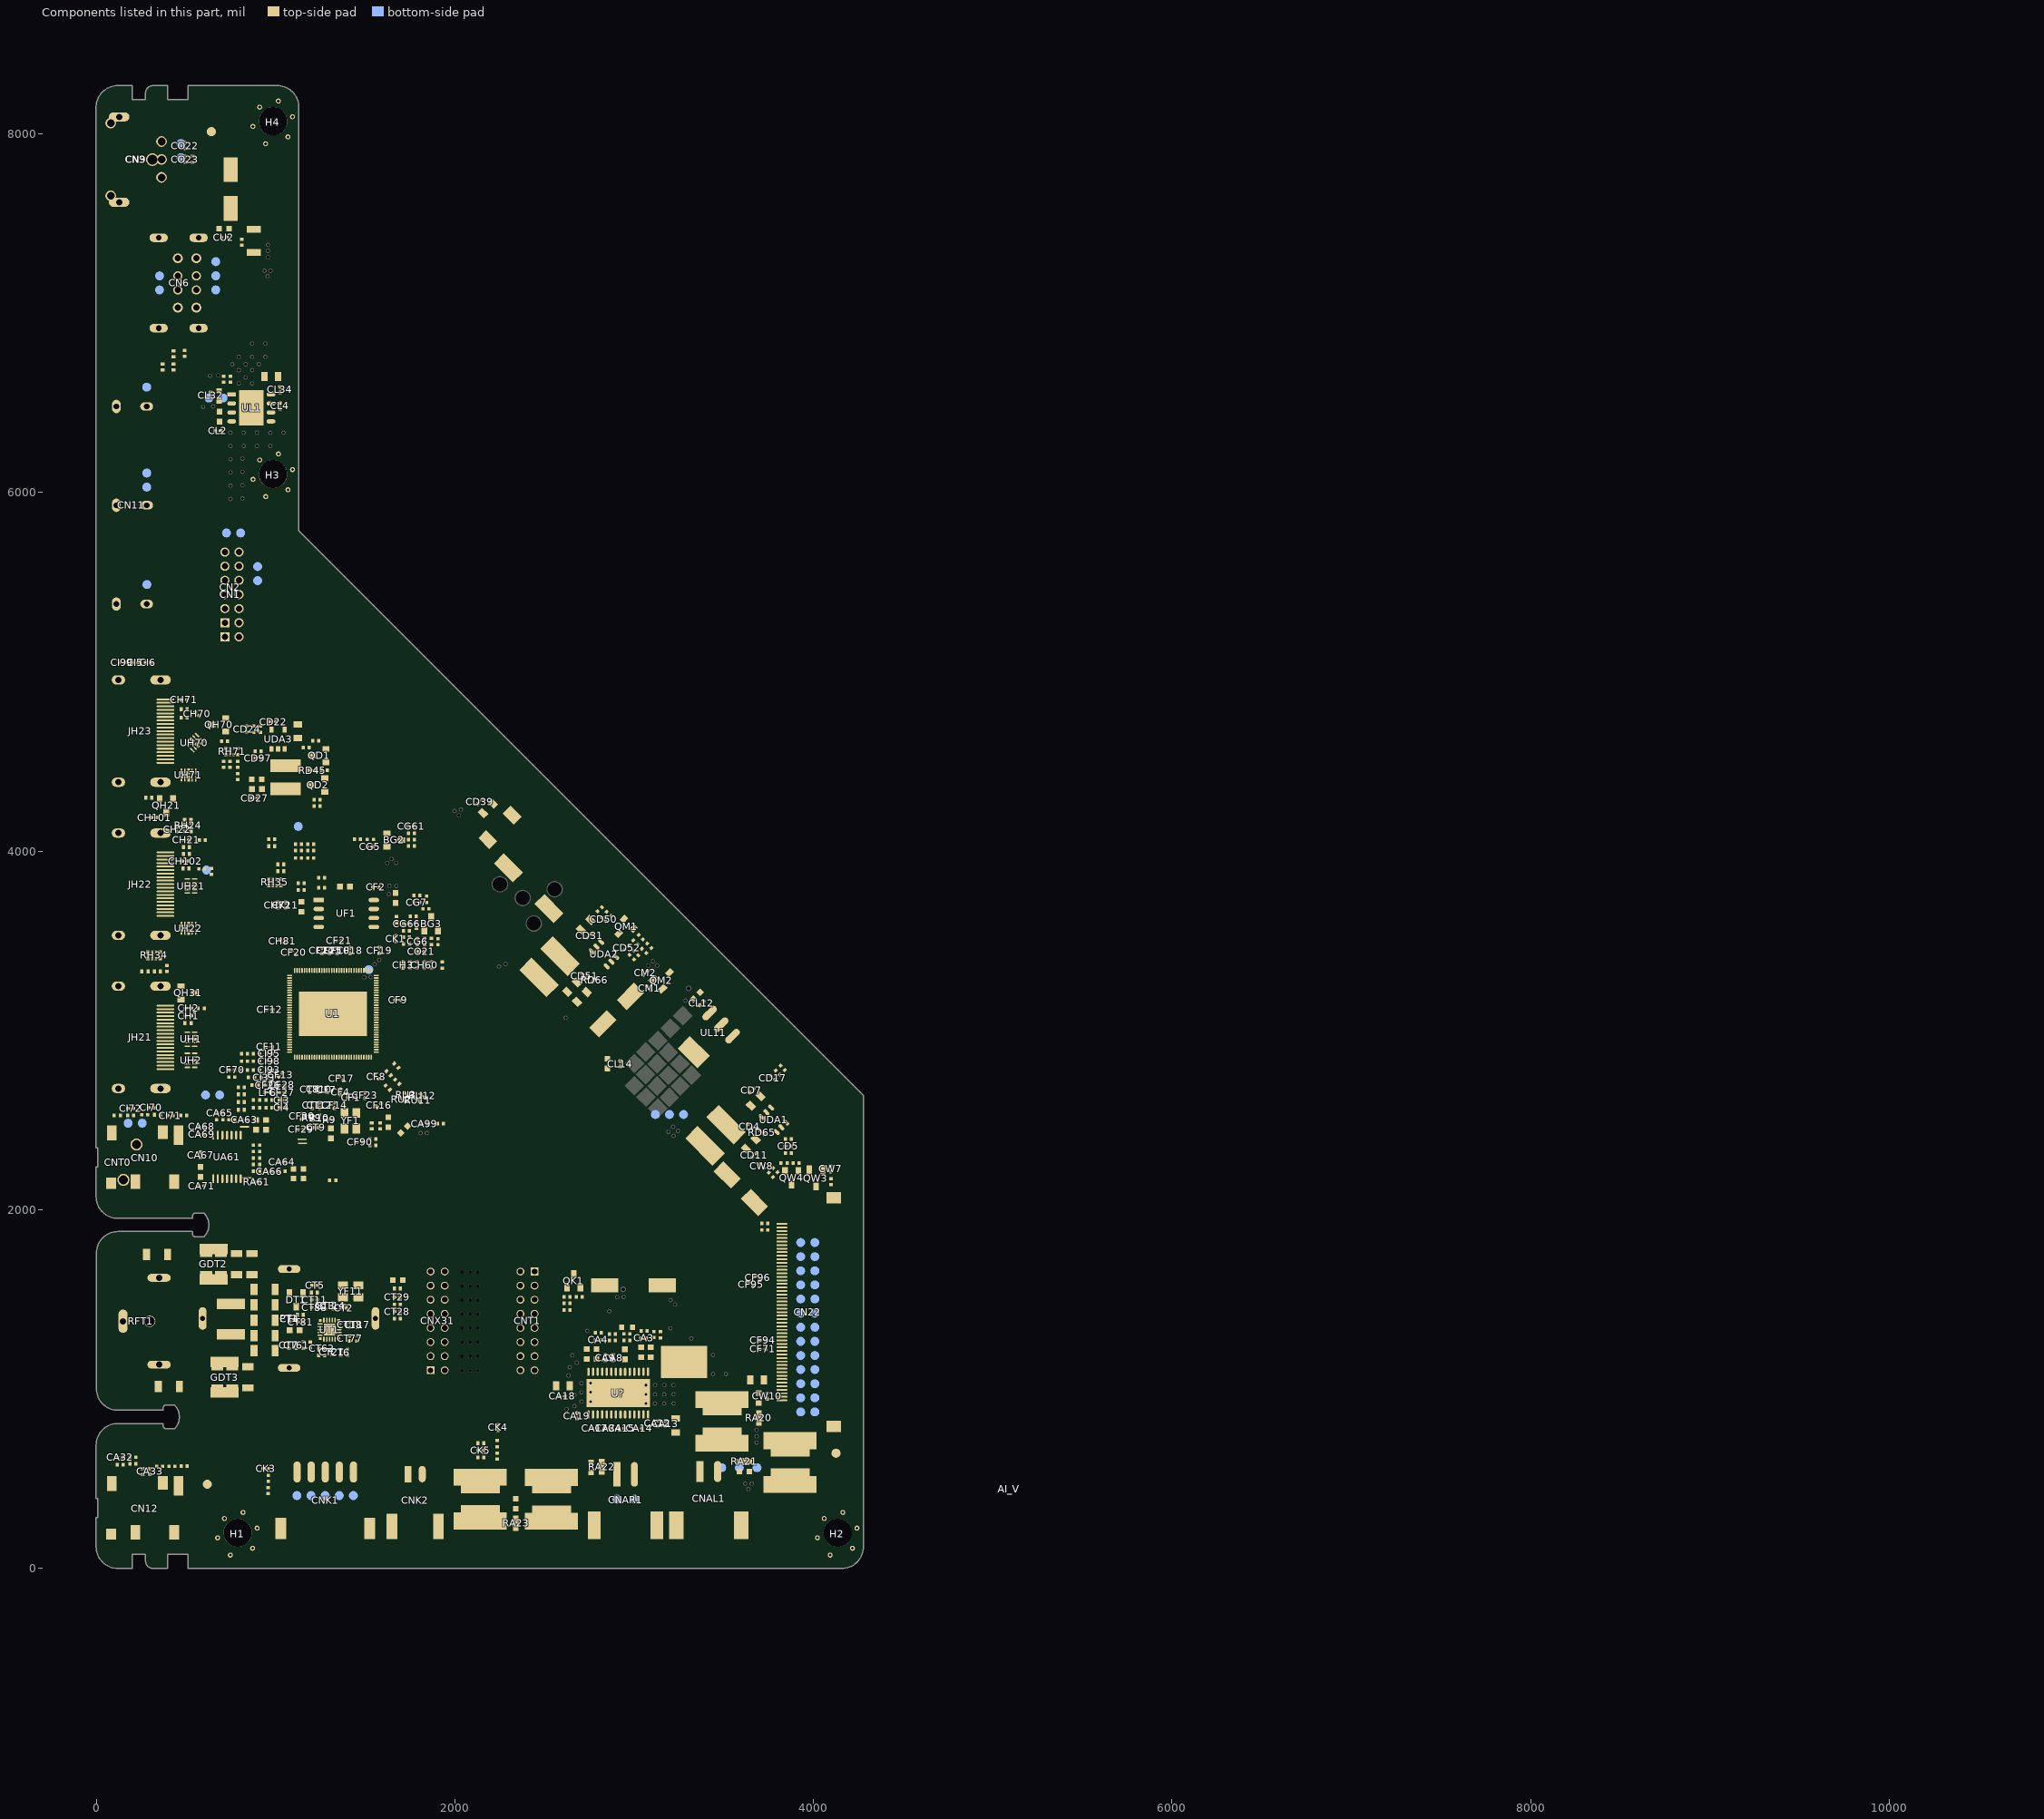
[diagram p0: the components of this part, seen from the top]
# Altium PCB MISC105950.PcbDoc (part 14 of 15)
Units mil, origin at the board's own origin, x right, y up, seen from the top; angles counter-clockwise.
Board outline 4280.62 x 8272.76 mil, 2 copper layers (TopLayer, BottomLayer), stack 61.855 mil thick; 541 components, 268 nets, 2324 pads, 1157 vias.

## Via types
v1: diameter 23.62, hole 15.75, TopLayer to BottomLayer, tented both sides, 1087 vias
v2: diameter 23.62, hole 15.75, TopLayer to BottomLayer, 51 vias
v3: diameter 27.56, hole 19.68, TopLayer to BottomLayer, 15 vias
v4: diameter 31.5, hole 19.68, TopLayer to BottomLayer, tented both sides, 4 vias

## Nets (pads, with @x,y where several pads share a name; then routed paths per layer and width w, separated by ;. In a path a pad name is that pad's centre, name@x,y a point inside that pad or via, vN(x,y) a via of type N, cw(c..) or ccw(c..) an arc to the next point about the centre after c; other vN are vias at no path point) (continued)
pads on no net: AI_V.0 AI_V.1 AI_V.2 CA3.2@3053,1282.5 CA4.2@2799.03,1273.23 CA8.2@2881.84,1172.5 CA9.2@2837.44,1172.5 CA12.2@3130.5,806.5 CA13.2@3173,806.16 CA14.2@3027,779 CA15.2@2929,779 CA17.2@2781,779 CA18.2@2598.5,958.5 CA19.2@2680,848.5 CA32.2@131.5,617 CA33.2@297,538.5 CA34.2@2855.5,779 CA63.2@824.76,2501 CA64.2@1035,2266 CA65.2@688,2539.5 CA66.2@962.73,2213.5 CA67.2@580,2304 CA68.2@585.66,2461.68 CA69.2@585.66,2420 CA71.2@585.34,2131.5 CA99.2@1829.34,2478.5 CD4.2@3643.54,2463.96 CD5.2@3858.27,2353.5 CD7.2@3654.54,2664.04 CD11.2@3669.5,2303.5 CD17.2@3773.5,2734.5 CD22.2@984.66,4721.5 CD24.2@838,4680.5 CD27.2@882.16,4295.5 CD31.2@2749,3527.51 CD39.2@2138.5,4274.5 CD50.2@2829,3619 CD51.2@2721.51,3302 CD52.2@2956.72,3460.11 CD97.2@900.77,4517.5 CF1.2@1417.66,2625 CF2.2@1558,3798 CF4.2@1361.5,2655.66 CF7.2@1285.5,2668.16 CF8.2@1561.5,2741.5 CF9.2@1681.5,3168.5 CF10.2@1341.5,3444.33 CF11.2@963.27,2907 CF12.2@965.5,3115.5 CF13.2@1026.5,2752 CF14.2@1326.5,2580.74 CF16.2@1575.96,2581.46 CF17.2@1365.5,2731.5 CF18.2@1414,3444.5 CF19.2@1577,3446 CF20.2@1099.67,3434.33 CF21.2@1352.16,3500.5 CF23.2@1497,2637.5 CF24.2@1257,3444.33 CF25.2@1299.5,3444.34 CF26.2@956,2693.5 CF27.2@1035,2652.5 CF28.2@1035,2694.5 CF29.2@1139.5,2447 CF30.2@1144.5,2520.23 CF70.2@755,2778 CF71.2@3716.5,1221.48 CF90.2@1469,2377 CF94.2@3716.5,1270.18 CF95.2@3650.86,1582.02 CF96.2@3688.61,1619.48 CG5.2@1525.5,4024 CG6.2@1789.5,3495.5 CG7.2@1786,3714 CG61.2@1754,4138.5 CG66.2@1729,3595 CH1.2@512.5,3081 CH2.2@512.5,3123 CH3.2@1709.5,3363.5 CH21.2@500.34,4062.1 CH22.2@449.5,4121.5 CH60.2@1828.5,3364.5 CH70.2@561.52,4764.99 CH71.2@488.5,4843.5 CH72.2@1011.5,3698.39 CH81.2@1037,3497 CH101.2@322.66,4187.5 CH102.2@493.83,3943.6 CI3.2@1034.99,2610 CI4.2@1034.99,2568 CI5.2@217,5052 CI6.2@288.5,5052 CI33.2@935.5,2736.5 CI70.2@305,2568.5 CI71.2@411,2524.5 CI72.2@190.5,2564 CI93.2@963.5,2778.5 CI95.2@963.5,2869 CI98.2@963.5,2827.5 CI99.2@143.5,5052 CK1.2@1670,3511 CK3.2@945,554.5 CK4.2@2240,784.5 CK5.2@2143,656.5 CK11.2@1053.5,3698.4 CL2.2@678,6345 CL4.2@1023.5,6483 CL12.2@3376,3150.5 CL14.2@2921.5,2813 CL32.2@635.42,6543.27 CL34.2@1023.5,6574.5 CM1.2@3082.7,3234.09 CM2.2@3061.5,3320 CN1.0 CN1.9 CN2.0 CN2.7 CN3.0 CN6.0 CN9.0 CN10.0 CN11.0 CN12.0 CN22.5 CN22.9 CN22.10 CN22.25 CN22.26 CN22.42 CN22.43 CN22.44 CN22.46 CN22.47 CN22.48 CN22.49 CN22.50 CN22.51 CNT0.0 CNT0.1 CNT1.0 CNT1.8 CNX31.0 CNX31.10 CO21.2@1811,3438.5 CO22.2@493,7935.37 CO23.2@493,7858.88 CT1.2@1201.5,2581.73 CT2.2@1377,1451 CT3.2@1276,1463 CT4.2@1077.5,1390.5 CT5.2@1217.5,1577 CT6.2@1361.5,1203.5 CT7.2@1072.5,1242.5 CT8.2@1189,2669.5 CT9.2@1223.34,2457 CT10.2@1241,2669.5 CT11.2@1214.98,1496.39 CT12.2@1244,2581.73 CT14.2@1318,1463 CT17.2@1455,1357.5 CT18.2@1412.5,1357.5 CT21.2@1313,1205.5 CT28.2@1678,1431.5 CT29.2@1677,1510.5 CT61.2@1114.5,1242.5 CT62.2@1256.5,1224.5 CT77.2@1412.5,1281.5 CT81.2@1137,1372.5 CT88.2@1214.99,1453.9 CU2.2@711,7423.88 CW7.2@4095.5,2227 CW8.2@3710.76,2241.97 CW10.2@3741.5,959 GDT2.1@613,1635.93 GDT2.1@654.98,1596.61 GDT2.1@693,1635.93 GDT2.2@613,1754.07 GDT2.2@654.98,1793.39 GDT2.2@693,1754.07 GDT3.1@674.5,1123.07 GDT3.1@712.52,1162.39 GDT3.1@754.5,1123.07 GDT3.2@674.5,1004.93 GDT3.2@712.52,965.61 GDT3.2@754.5,1004.93 H1.0 H2.0 H3.0 H4.0 JH21.0 JH22.0 JH23.0 JH23.14 M1.0 M2.0 M3.0 Manufacture_Info.0 PT1.0 RFT1.0 S/N1.0 S/N2.0 U1.0 U?.13 U?.EPAD UT1.1 UT1.9 UT1.10 UT1.15 XX.XXXX.0 XXXXXX.0 XXXXXX..0 XXXXXXXX.0 XXXXXXXXXX.0 用U1上.0
copper on no net: | length 3400.6
  TopLayer w5: 8224.49,3310.69 8224.49,3389.43 ; 7673.59,3310.69 8405.62,3310.69 8405.62,3389.43 7673.59,3389.43 7673.59,3310.69
  BottomLayer w5: 8224.49,3092.84 8224.49,3171.58 ; 7673.59,3092.84 7673.59,3171.58 8405.62,3171.58 8405.62,3092.84 7673.59,3092.84
  other v1: 2737.24,898.49 2816.34,898.27 2879.33,898.27 2942.33,898.27 3006.33,898.27 3083.17,898.49 2737.24,936.95 3083.17,936.95 2737.24,975.41 3083.17,975.41 2737.24,1013.86 3083.17,1013.86 2737.24,1052.32 2816.34,1052.09 2879.33,1052.09 2942.33,1052.09 3006.33,1052.1 3083.17,1052.32
  other v3: 2783.2,922.26 2847.21,922.26 2910.2,922.26 2973.2,922.26 3037.2,922.26 2783.2,975.41 2847.21,975.41 2910.2,975.41 2973.2,975.41 3037.2,975.41 2783.2,1028.56 2847.21,1028.56 2910.2,1028.56 2973.2,1028.56 3037.2,1028.56

## Polygon pours and split planes (outlines as drawn)
GND on BottomLayer "5" (solid, remove dead copper, pour order 22): 1135.5,5505 1092,5461.5 883.5,5461.5 883,5461.5 853.5,5432 853.5,5368 897,5324.5 897,5074.5 873.5,5051 541,4718.5 541,4636 345,4636 168,4459 168,2786 467,2487 768,2487 951.5,2303.5 1112.5,2142.5 1112.5,2074 1151.5,2074 1204.5,2021 1650.83,2021 1680.17,2050.33 1734.5,2104.67 1734.5,2170.5 1781.5,2217.5 2038,2217.5 2203.5,2052 2203.5,1699.5 2203.5,898 2249.5,852 2339.5,852 2774,1286.5 2774,1449 2852,1527 2852,1535.65 2875.58,1559.22 2900.35,1584 2946.5,1584 2987,1584 3093.5,1690.5 3121,1718 3121,1758.5 3121,2412.67 3170.16,2461.83 3159.5,2472.49 3159.5,2570 3159.5,2648.5 3296,2785 3395.5,2685.5 3454.5,2685.5 3454.5,2649.5 3751,2353 3849,2451 3951.5,2451 3951.5,2689 3959,2696.5 1161.5,5494 1161.5,5525
GND on BottomLayer "5" (solid, remove dead copper, pour order 23): 1873,2503.5 1745.5,2503.5 1725,2524 1703,2546 1703,2573 1703,2595 1732,2624 1734,2626 1779,2626 1782,2626 1810.5,2654.5 2029,2873 2029,3070.5 2029,3447 2124.5,3542.5 2146.31,3564.31 2216.93,3564.31 2277.5,3503.74 2277.5,3441 2277.5,3404.5 2254,3381 2202.5,3381 2190.5,3369 2181.5,3360 2181.5,3238 2181.5,2834 2038,2690.5 1945.67,2598.17 1945.67,2572 1945.67,2544.19 1928.79,2527.31 1904.98,2503.5 1873,2503.5
RFGND on BottomLayer "12" (solid, remove dead copper, pour order 18): 217.5,1908 71,1908 -6.5,1830.5 -6.5,929 56,866.5 271,866.5 328,923.5 467.5,1063 606.5,1063 890,1063 936.5,1109.5 936.5,1652.5 904,1685 465,1685 394.5,1755.5 273,1877 268,1877
GND on BottomLayer "12" (solid, remove dead copper, pour order 19): 67.5,2492.5 1238,2492.5 1750,1980.5 1750,1235 1127,612 1115.5,600.5 815.5,600.5 381,600.5 298.5,683 298.5,878.5 459,1039 873,1039 938,1104 938,1663 928,1673 458,1673 301,1830 225,1906 -57,1906 -57,1966.5 -171,2080.5
GND on BottomLayer "12" (solid, remove dead copper, pour order 20): 596.5,8267.72 100,8267.72 ccw(c100,8167.72) 0,8167.72 0,8129 0,2053.33 ccw(c100,2053.33) 100,1953.33 294,1953.33 294,1852 443.5,1702.5 903.82,1702.5 948.07,1658.25 948.07,1124.07 900,1076 482.5,1076 382.5,976 199,792.5 172,792.5 82.92,792.5 ccw(c82.92,692.5) 12.21,763.21 2,753 ccw(c11.66,743.34) -2,743.34 -2,644.5 -2,100 ccw(c98,100) 98,0 145.5,0 4173.75,0 ccw(c4173.75,100) 4273.75,100 4273.75,334.08 4273.75,2638.25 4101.5,2810.5 1125.98,5786.02 1125.98,6061 1125.98,8167.78 ccw(c1025.98,8167.78) 1025.98,8267.78 994,8267.78 553.5,8267.78
GND on BottomLayer "5" (solid, remove dead copper, pour order 21): 4064.5,1940 3740.5,1940 3633,1832.5 3637,1828.5 3637,1821 3637,1041 3932,746 3940.5,737.5 4103.5,737.5 4103.5,838.5 4140.5,875.5 4130,886 4130,1964.5
GND on TopLayer "12" (solid, remove dead copper, pour order 15): 596.5,8267.72 100,8267.72 ccw(c100,8167.72) 0,8167.72 0,8129 0,2053.33 ccw(c100,2053.33) 100,1953.33 294,1953.33 294,1852 443.5,1702.5 903.82,1702.5 948.07,1658.25 948.07,1124.07 900,1076 482.5,1076 382.5,976 199,792.5 172,792.5 82.92,792.5 ccw(c82.92,692.5) 12.21,763.21 2,753 ccw(c11.66,743.34) -2,743.34 -2,644.5 -2,100 ccw(c98,100) 98,0 145.5,0 4173.75,0 ccw(c4173.75,100) 4273.75,100 4273.75,334.08 4273.75,2638.25 4101.5,2810.5 1125.98,5786.02 1125.98,6061 1125.98,8167.78 ccw(c1025.98,8167.78) 1025.98,8267.78 994,8267.78 553.5,8267.78
RFGND on TopLayer "12" (solid, remove dead copper, pour order 17): 889.86,1695.63 468.87,1695.63 343,1821.5 271,1893.5 72,1893.5 38,1893.5 18,1873.5 1.21,1856.71 1.21,1532.5 1.21,910.79 40.5,871.5 51.47,882.47 219,882.47 315.97,882.47 365.5,932 481.5,1048 695.5,1048 882.5,1048 924.5,1090 938,1103.5 938,1574 938,1650.71 943.75,1656.46 904.59,1695.63 889.86,1695.63
GND on TopLayer "5" (solid, remove dead copper, pour order 16): 507,4715.33 449.83,4715.33 435.5,4701 435.5,4456.5 442.5,4449.5 442.5,4303.5 485.5,4260.5 670.66,4075.34 670.66,3880 669,3880 657.5,3868.5 652.56,3863.56 448.47,3863.56 444.4,3863.56 435.16,3854.33 435.16,3636.84 423,3624.68 423,3623.88 431.33,3615.56 452.48,3594.41 452.48,3564.5 452.48,3467.89 557.59,3362.78 652,3268.37 652,3120 652,3076.36 598.64,3023 586.52,3010.88 462.88,3010.88 446.04,3010.88 435.16,3000 435.16,2774.01 431,2769.85 433.03,2771.87 487,2771.87 640.69,2771.87 690.81,2822 775.81,2907 785,2907 884,2907 885.5,2905.5 956.47,2905.5 999.83,2948.86 1056.5,3005.53 1056.5,3084.99 1056.5,3291.04 1087.25,3321.79 1099.49,3334.04 1104.92,3334.04 1126.19,3355.31 1126.19,3379.5 1126.19,3392.5 1126.19,3407.81 1048.83,3485.17 1048.83,3498.73 1009.14,3538.42 883.5,3664.07 883.5,3858.5 883.5,4213.48 880,4216.98 866.84,4230.14 866.84,4235.3 709.78,4392.36 676.33,4392.36 676.33,4560.95 623.51,4613.76 515.6,4721.67 485.37,4721.67
GND on TopLayer "5" (solid, remove dead copper, pour order 13): 342.07,7337 306.59,7337 111.81,7142.22 111.81,6802.69 225.5,6689 288,6689 320.5,6656.5 320.5,5075.04 615.04,4780.5 1108,4780.5 1251.21,4637.29 1343.99,4637.29 1396.69,4584.6 1402.81,4584.6 1402.81,4542.19 1771,4174 1833.53,4174 2046.76,3960.76 2046.76,3749.24 2089,3707 2089,3479 2158.5,3409.5 2247,3409.5 2259,3421.5 2259,3680.5 2159,3780.5 2159,3993.67 1203.17,4949.5 648.5,4949.5 475,5123 475,6580 527,6632 527,6820.5 500,6847.5 293.5,6847.5 254,6887 254,7047.43 258.66,7052.09 336.09,7052.09 375,7091 375,7317 354.56,7337.44 341.44,7337.44
GND on TopLayer "5" (solid, remove dead copper, pour order 14): 1633.94,3293.19 1633.94,3279.02 1576.5,3221.58 1576.5,2893.5 1563,2880 1541.36,2880 1536.17,2885.18 1504.52,2853.54 1504.52,2793.64 1602.83,2695.33 1602.83,2688.57 1769.93,2521.47 1948.68,2521.47 1963.3,2506.84 2069.97,2506.84 2167.89,2408.92 2205.25,2408.92 2813.45,1800.72 2899.78,1800.72 3045.5,1655 3057.5,1655 3057.5,1625.7 3102.95,1580.24 3102.95,1502.55 3122.96,1522.55 3235.95,1522.55 3657.06,1101.44 3703.5,1101.44 3716.44,1088.5 3762,1088.5 3778.96,1071.54 3778.96,1014.84 3800.66,1014.84 3870,945.5 4003,945.5 4116.5,1059 4116.5,1751.5 3996.5,1871.5 3918.42,1871.5 3865.85,1818.93 3865.85,1741.35 3845.5,1721 3796.61,1721 3781.9,1735.71 3783.63,1737.44 3783.63,1801.37 3775.5,1809.5 3775.5,1839.45 3754.93,1860.03 3720.71,1860.03 3224.59,2356.15 3145.35,2356.15 2267.1,3234.4 2213.19,3234.4 2171.88,3275.72 2129.78,3275.72 2068.2,3337.3 1968.03,3337.3 1951.23,3320.5 1645.25,3320.5 1633.94,3309.19 1633.94,3293.19

## Keep-outs
KeepOutLayer:
  circle w2.5: c118.11,8267.73 r1.25
  circle w2.5: c4275.59,118.11 r1.25
  circle w2.5: c1185.04,8326.78 r1.25
  circle w2.5: c5342.52,177.16 r1.25
  rectangle: 7673.59,2713.41 7803.79,2792.15
  lines w5: 0,2346 7.42,2346 7.87,2345.54 7.87,2236.22 0,2236.22 0,2071.44 ccw(c118.11,2071.44) 118.11,1953.33 532,1953.33 ; 0,2346.46 0,8153 ; 0,8149.62 cw(c118.11,8149.62) 118.11,8267.73 196.85,8267.73 196.85,8188.99 275.59,8188.99 275.59,8228.36 cw(c314.96,8228.36) 314.96,8267.73 393.7,8267.73 393.7,8188.99 511.81,8188.99 511.81,8267.73 1008.03,8267.72 ; 368.5,803.73 118.11,803.73 ccw(c118.11,685.62) 0,685.62 0,389.76 7.87,389.76 7.87,279.53 0,279.53 0,118.11 ccw(c118.11,118.11) 118.11,0 196.85,0 196.85,78.74 275.59,78.74 275.59,39.37 ccw(c314.96,39.37) 314.96,0 393.7,0 393.7,78.74 511.81,78.74 511.81,0 4157.48,0 ccw(c4157.48,118.11) 4275.59,118.11 4275.59,2576.35 4275.59,2635.41 1125.98,5785.02 1125.98,8149.61 ccw(c1007.87,8149.61) 1007.87,8267.72 ; 368.5,882.47 119.32,882.47 cw(c119.32,1000.58) 1.21,1000.58 1.21,1756.48 cw(c119.32,1756.48) 119.32,1874.59 532,1874.59 ; 368.7,803.32 368.7,793.82 ccw(c388.39,793.82) 388.39,774.14 436.03,774.14 ccw(c367.13,843.03) 436.03,911.93 388.39,911.93 ccw(c388.39,892.25) 368.7,892.25 368.7,882.47 ; 396.88,2108.85 235.46,2108.85 ; 532.7,1874.59 532.7,1864.75 ccw(c552.39,1864.75) 552.39,1845.07 600.03,1845.07 ccw(c531.13,1913.96) 600.03,1982.86 552.39,1982.86 ccw(c552.39,1963.18) 532.7,1963.18 532.7,1953.33 ; 640.2,774.14 687.84,774.14 ccw(c618.94,843.03) 687.84,911.93 640.2,911.93 ; 642.72,774.14 595.08,774.14 cw(c663.98,843.03) 595.08,911.93 642.72,911.93 ; 708.54,8267.72 ccw(c679.01,8297.25) 708.54,8326.78 ; 826.41,1874.59 826.41,1864.75 cw(c806.72,1864.75) 806.72,1845.07 759.08,1845.07 cw(c827.98,1913.96) 759.08,1982.86 806.72,1982.86 cw(c806.72,1963.18) 826.41,1963.18 826.41,1953.33 ; 826.5,1874.59 1922.47,1874.59 cw(c1922.47,1756.48) 2040.58,1756.48 2040.58,1740 ; 826.5,1953.33 2048.46,1953.33 cw(c2048.46,1874.59) 2127.2,1874.59 ; 914.22,803.71 914.22,793.82 cw(c894.53,793.82) 894.53,774.14 846.89,774.14 cw(c915.79,843.03) 846.89,911.93 894.53,911.93 cw(c894.53,892.25) 914.22,892.25 914.22,882.46 ; 915.5,803.71 2048.44,803.71 ccw(c2048.46,882.47) 2127.2,882.47 2126.93,882.74 2126.93,1016.5 ccw(c2083.78,973.35) 2040.63,1016.5 2040.58,1000.5 ; 915.5,882.47 1922.47,882.47 ; 993.88,8267.72 cw(c1023.41,8297.25) 993.88,8326.78 ; 1125.98,7500.79 cw(c1155.51,7471.26) 1185.04,7500.79 ; 1125.99,7943.61 ccw(c1155.51,7973.14) 1185.04,7943.61 ; 1662.12,5248.86 ccw(c1662.12,5290.62) 1703.88,5290.62 ; 1670.27,5324.25 3408.51,3586.01 ; 1753.78,5157.22 3467.62,3443.38 ; 1975.24,4935.74 cw(c2017,4935.74) 2017,4977.5 ; 2040.63,1740.57 ccw(c2083.78,1783.72) 2126.93,1740.57 2127.2,1740.84 2127.2,1769.74 ; 3412.18,7641.16 ccw(c3412.18,7562.42) 3333.44,7562.42 3333.44,6675.15 3333.44,6570.29 ccw(c3412.18,6570.29) 3412.18,6491.55 4870.45,6491.55 4870.45,6481.71 ccw(c4890.13,6481.71) 4890.13,6462.02 4937.77,6462.02 ccw(c4868.87,6530.92) 4937.77,6599.82 4890.13,6599.82 ccw(c4890.13,6580.13) 4870.45,6580.13 4870.45,6570.29 3538.16,6570.29 cw(c3538.16,6688.4) 3420.05,6688.4 3420.05,7444.31 ; 3412.19,7641.17 4870.45,7641.17 4870.45,7651.06 cw(c4890.13,7651.06) 4890.13,7670.75 4937.77,7670.75 cw(c4868.87,7601.85) 4937.77,7532.95 4890.13,7532.95 cw(c4890.13,7552.64) 4870.45,7552.64 4870.45,7562.43 ; 3420.05,7444.39 cw(c3538.16,7444.31) 3538.16,7562.42 4870.45,7562.42 ; 3443.63,3467.39 ccw(c3443.63,3509.14) 3485.39,3509.14 ; 3756.75,3154.27 cw(c3798.51,3154.27) 3798.51,3196.02 ; 4275.59,501.28 cw(c4305.12,471.75) 4334.65,501.28 ; 4275.59,944.1 ccw(c4305.12,973.62) 4334.65,944.1 ; 4452.6,177.17 4948.82,177.17 4948.82,255.9 5066.93,255.9 5066.93,177.16 5145.67,177.16 ccw(c5145.67,216.53) 5185.04,216.53 5185.04,255.9 5263.78,255.9 5263.78,177.16 5342.52,177.16 ccw(c5342.52,295.27) 5460.63,295.27 ; 4452.76,177.17 cw(c4452.76,295.28) 4334.65,295.28 4334.65,2659.87 1185.04,5809.48 1185.04,5868.53 1185.04,8326.78 cw(c1303.15,8326.78) 1303.15,8444.89 4948.82,8444.89 4948.82,8366.15 5066.93,8366.15 5066.93,8444.89 5145.67,8444.89 cw(c5145.67,8405.52) 5185.04,8405.52 5185.04,8366.15 5263.78,8366.15 5263.78,8444.89 5342.52,8444.89 cw(c5342.52,8326.78) 5460.63,8326.78 5460.63,8165.36 5452.76,8165.36 5452.76,8055.12 5460.63,8055.12 5460.63,7759.27 cw(c5342.52,7759.27) 5342.52,7641.16 5164.13,7641.16 ; 4466.76,118.11 ccw(c4437.23,147.64) 4466.76,177.17 ; 4752.09,118.11 cw(c4781.62,147.64) 4752.09,177.17 ; 5164.15,6491.55 5164.15,6481.71 cw(c5144.46,6481.71) 5144.46,6462.02 5096.83,6462.02 cw(c5165.72,6530.92) 5096.83,6599.82 5144.46,6599.82 cw(c5144.46,6580.13) 5164.15,6580.13 5164.15,6570.29 5341.31,6570.29 ccw(c5341.31,6688.4) 5459.42,6688.4 5459.42,7444.31 ccw(c5341.31,7444.31) 5341.31,7562.42 5164.15,7562.42 5164.15,7552.64 cw(c5144.46,7552.64) 5144.46,7532.95 5096.83,7532.95 cw(c5165.72,7601.85) 5096.83,7670.75 5144.46,7670.75 cw(c5144.46,7651.06) 5164.15,7651.06 5164.15,7641.57 ; 5165.36,6491.55 5342.52,6491.55 cw(c5342.52,6373.44) 5460.63,6373.44 5460.63,6208.66 5452.76,6208.66 5452.76,6099.34 5453.22,6098.89 5460.63,6098.89 ; 5460.63,291.89 5460.63,6098.43 ; 8224.49,2713.41 8224.49,2792.15 ; 235.46,2108.85 396.88,2108.85 396.88,2030.11 235.46,2030.11 235.46,2108.85 ; 865.38,2108.85 1026.8,2108.85 ; 865.38,2108.85 865.38,2030.11 1026.8,2030.11 1026.8,2108.85 ; 865.38,2108.85 1026.8,2108.85 ; 1849.64,2108.85 2011.05,2108.85 ; 1849.64,2108.85 1849.64,2030.11 2011.05,2030.11 2011.05,2108.85 ; 1849.64,2108.85 2011.05,2108.85 ; 1922.47,882.47 ccw(c1922.47,1000.58) 2040.58,1000.5 ; 1922.47,882.47 ccw(c1922.47,1000.58) 2040.58,1000.5 ; 2127.2,1769.74 2127.2,1874.59 ; 2127.2,1769.74 2127.2,1874.59 ; 3449.58,6336.04 3611,6336.04 ; 3449.58,6336.04 3611,6336.04 ; 3449.58,6336.04 3449.58,6414.78 3611,6414.78 3611,6336.04 ; 4334.65,118.11 5460.63,118.11 ; 4334.65,118.11 4334.65,19.69 ccw(c4354.33,19.69) 4354.33,0 5440.95,0 ccw(c5440.95,19.69) 5460.63,19.69 5460.63,118.11 ; 4334.65,118.11 5460.63,118.11 ; 4433.83,6336.04 4595.25,6336.04 ; 4433.83,6336.04 4595.25,6336.04 ; 4433.83,6336.04 4433.83,6414.78 4595.25,6414.78 4595.25,6336.04 ; 5063.75,6336.04 5225.17,6336.04 ; 5063.76,6336.04 5225.17,6336.04 ; 5063.76,6336.04 5063.76,6414.78 5225.17,6414.78 5225.17,6336.04 ; 0,8326.78 0,8425.2 cw(c19.68,8425.2) 19.68,8444.89 1106.3,8444.89 cw(c1106.3,8425.2) 1125.99,8425.2 1125.98,8326.78 0,8326.78 ; 235.46,648.21 396.88,648.21 396.88,726.95 235.46,726.95 235.46,648.21 ; 865.38,648.21 1026.8,648.21 1026.8,726.95 865.38,726.95 865.38,648.21 ; 1849.64,648.21 2011.05,648.21 2011.05,726.95 1849.64,726.95 1849.64,648.21 ; 3449.58,7717.93 3449.58,7796.67 3611,7796.67 3611,7717.93 3449.58,7717.93 ; 4433.83,7717.93 4433.83,7796.67 4595.25,7796.67 4595.25,7717.93 4433.83,7717.93 ; 5063.76,7717.93 5063.76,7796.67 5225.17,7796.67 5225.17,7717.93 5063.76,7717.93 ; 7673.59,2713.41 7673.59,2792.15 8405.62,2792.15 8405.62,2713.41 7673.59,2713.41
  text "KeepOutLayer" at 7826.39,2734.37 h60
  text ".GKO" at 8248.2,2731.46 h60

## Other copper
TopLayer:
  drawing of 341 lines, arcs and shapes, not listed
  text "TopLayer" at 7839.64,3333.03 h60
  text ".GTL" at 8249.13,3328.74 h60
BottomLayer:
  rectangle net GND: 650,2588 727,2686
  rectangle net GND: 1237,356 1313,467
  rectangle: 7673.59,3092.84 7803.79,3171.58
  rectangle net GND: 3400.5,504 3525.5,661
  rectangle net GND: 3972,825 4080,906
  rectangle net GND: 982,1041 1246.5,1209
  rectangle net GND: 980.5,1567 1247.5,1766
  rectangle net GND: 196.5,6070 358.5,6168
  rectangle net GND: 35,7579 221,7716
  rectangle net GND: 314.5,7683.5 426.5,7789.5
  pour cut-out: 378.5,947 378.5,945.77 433.5,890.77 433.5,885 358.5,885 357,886.5
  pour cut-out: 313,1895 315,1897 419,1897 419,1890 398.5,1869.5 415.5,1869.5 394,1848 394,1794 392.5,1792.5 369,1816 337.5,1816
  region net VDDC_CORE: 1626,3891 1626,3909 1608,3927 1608,3941 1613,3946 1634,3946 1634,3943 1650,3927
  pour cut-out: 721.13,1647.86 923.86,1647.86 931,1655 931,1704 908.55,1726.45 468.45,1726.45 452,1710 452,1660 463.54,1648.46 725.75,1648.46
  region net 12V/15V: 3210,1467 3218,1459 3234,1459 3239,1464 3239,1479 3232,1486
  pour cut-out: 736.3,1723.3 703.6,1723.3 698.7,1718.4 715.4,1701.7 723.3,1701.7 741.9,1720.3
  pour cut-out: 757.3,1657.4 749,1649.1 726.4,1649.1 726.4,1650.4 712.4,1664.4 759.3,1664.4
  pour cut-out: 452.8,7373.8 350.6,7373.8 303.1,7326.3 303.1,7076.1 337.8,7041.4 601.4,7041.4 607.8,7047.8 607.8,7349.8 584.3,7373.3 459.8,7373.3
  pour cut-out: 847.8,1690.8 893.6,1690.8 932.6,1651.8 932.6,1600.6 850.5,1682.7 850.5,1689.3
  region net VDDC_CORE: 1645.5,3969 1657.5,3969 1681.5,3945 1681.5,3796 1634.26,3748.76 1625.32,3748.76 1615,3759.09 1615,3777.5 1621.09,3783.59 1621.09,3944.59
  region net LOUT+: 3618,428 3607,439 3607,471.5 3667.5,532 3684.19,532 3684.19,468.69 3643.5,428
  region net VDDC_CORE: 1581.5,3404.5 1551.5,3404.5 1486.5,3339.5 1486.5,3289.5 1492.5,3283.5 1534.5,3283.5 1542.5,3291.5 1542.5,3327.5 1588.5,3373.5 1588.5,3397.5
  region net 12V/15V: 3047,1494.5 3059.5,1507 3227.5,1507 3236,1498.5 3236,1467.5 3230,1461.5 3049,1461.5 3045.5,1465
  pour cut-out: 411.75,861.54 411.75,970.25 417,975.5 359.5,975.5 359.5,910.5 365.5,904.5
  region net GND: 1476.5,1497.5 1476.5,1349.5 1534,1292 1598,1292 1628,1322 1628,1390.24 1595.19,1423.05 1595.19,1473.81 1562.5,1506.5 1560,1506.5
  region net GND: 2243,1700 2243,1010.89 2222.61,990.5 2222.61,1679.61
  pour cut-out: 998.14,3998.5 998.14,3967.1 1020.5,3944.74 1020.5,3939.43 1013,3939.43 1009.61,3942.81 953.19,3942.81 941.5,3954.5
  pour cut-out: 1041,3931.78 984.03,3931.78 969.35,3917.1 969.35,3937.46 964,3942.81
  pour cut-out: 3205.4,2494.45 3237.06,2494.45 3252.59,2478.92 3263.5,2489.83 3263.5,2503.5 3247.5,2519.5
  pour cut-out: 1854.5,3770.86 1849.8,3766.16 1816.56,3766.16 1816.56,3775.44 1810,3782 1822.56,3794.56 1838.66,3794.56
  pour cut-out: 1792.86,3782 1792.86,3791.4 1776.88,3807.38 1796,3826.5 1810,3826.5
  pour cut-out: 1767.56,3916.34 1767.56,3957.06 1747.88,3937.38 1747.88,3908.7 1744.9,3905.72 1750.12,3900.5 1761,3900.5
  pour cut-out: 1901.34,4062.94 1901.34,4017.52 1893.31,4009.5 1876.52,4026.29 1876.52,4027.84
  pour cut-out: 585.5,3991.14 591.9,3991.14 609.38,4008.62 621.5,3996.5 609.38,3984.38
  pour cut-out: 568.36,3974 568.36,3927.64 575.22,3934.5 597.5,3934.5
  pour cut-out: 571.88,3921.88 571.88,3898.06 583.77,3886.17 602.6,3905 613,3905
  pour cut-out: 382.21,4157.59 382.21,4150.83 402.85,4130.19 433.5,4130.19 433.5,4146.11 431.59,4148.02
  pour cut-out: 291.5,4240.36 314.4,4240.36 319.38,4235.38 331.5,4247.5 331.5,4264.81 333.5,4266.81
  pour cut-out: 1040.84,4181.56 1040.84,4164.54 1065.73,4139.65 1048.16,4122.07 1040.93,4122.07 1025,4138
  pour cut-out: 961.5,4170.64 999.9,4170.64 1008.75,4179.5 1008.75,4167.91 1011.05,4165.62
  pour cut-out: 1095.77,4129.67 1096.16,4129.28 1096.16,4089.53 1109.77,4103.14 1112,4103.14
  pour cut-out: 2248.59,1952.55 2281.16,1919.97 2281.16,1908.56 2309.32,1908.56 2311.43,1910.67 2310.5,1911.59 2310.5,1953.5
  pour cut-out: 2290.75,1893.74 2290.75,1855.75 2307.25,1872.26
  region net GND: 438,7761.5 395,7804.5 352,7804.5 344,7796.5 341,7796.5 341,7796.3 332.59,7787.89 425.48,7695 438,7695
  region net 5V_M: 938.34,7258.34 924.1,7244.1 924.1,7215.9 944.1,7195.9 960.9,7195.9 985,7220 985,7240 966.35,7258.65
  region net 5V_M: 3083,3338 3097,3324 3121.27,3324 3139.86,3342.6 3139.86,3365.14 3128,3377 3113,3377
  pour cut-out: 3941,1725 3941,1667 3899,1625 3889,1625 3888,1624 3888,1670 3936,1718
  pour cut-out: 301.57,837.43 cw(c276.5,862.5) 251.43,887.57 300.87,937 300.83,936.96 cw(c325.93,911.93) 306.55,941.61 459.5,1094.57 459.47,1094.53 cw(c484.57,1069.5) 484.57,1104.95 895.32,1104.95 901.55,1111.18 901.55,1664.32 899.93,1665.93 cw(c925,1691) 950.07,1716.07 962.07,1704.07 962.03,1704.1 cw(c937,1679) 972.45,1679 972.45,1096.5 cw(c937,1096.5) 962.03,1071.4 962.07,1071.43 935.07,1044.43 935.1,1044.47 cw(c910,1069.5) 910,1034.05 499.25,1034.05 352.07,886.87 352.1,886.9 cw(c327,911.93) 346.38,882.25
  pour cut-out: 435.93,1657.93 231.93,1861.93 cw(c257,1887) 282.07,1912.07 475.68,1718.45 714.07,1718.45 cw(c736.5,1691) 736.5,1726.45 934.5,1726.45 cw(c934.5,1691) 969.95,1691 cw(c934.5,1691) 934.5,1655.55 738.93,1655.55 cw(c716.5,1683) 716.5,1647.55 461,1647.55 cw(c461,1683)
  pour cut-out: 583.18,7369.4 701.1,7369.4 cw(c701.1,7324.5) 746,7324.5 746,7151.45 cw(c646,7151.45) 646,7051.45 561.55,7051.45 cw(c561.55,7103.5) 509.5,7103.5 509.5,7137.5 cw(c526,7137.5) 526,7154
  pour cut-out: 366,7275 316.5,7275 ccw(c316.5,7260) 301.5,7260 301.5,7085 ccw(c339,7085) 339,7047.5 509.5,7047.5 ccw(c509.5,7068) 530,7068 530,7109.5 ccw(c524,7109.5) 524,7115.5 cw(c524,7175.5) 464,7175.5 464,7279
  pour cut-out: 2018,1081.62 2145,1081.62 ccw(c2145,1101.32) 2164.7,1101.32 ccw(c2145,1101.32) 2145,1121.02 2018,1121.02 ccw(c2018,1101.32)
  pour cut-out: 2018,1160.36 2145,1160.36 ccw(c2145,1180.06) 2164.7,1180.06 ccw(c2145,1180.06) 2145,1199.76 2018,1199.76 ccw(c2018,1180.06)
  pour cut-out: 2018,1239.1 2145,1239.1 ccw(c2145,1258.8) 2164.7,1258.8 ccw(c2145,1258.8) 2145,1278.5 2018,1278.5 ccw(c2018,1258.8)
  pour cut-out: 2018,1317.84 2145,1317.84 ccw(c2145,1337.54) 2164.7,1337.54 ccw(c2145,1337.54) 2145,1357.24 2018,1357.24 ccw(c2018,1337.54)
  pour cut-out: 2018,1396.58 2145,1396.58 ccw(c2145,1416.28) 2164.7,1416.28 ccw(c2145,1416.28) 2145,1435.98 2018,1435.98 ccw(c2018,1416.28)
  pour cut-out: 2018,1475.32 2145,1475.32 ccw(c2145,1495.02) 2164.7,1495.02 ccw(c2145,1495.02) 2145,1514.72 2018,1514.72 ccw(c2018,1495.02)
  pour cut-out: 2018,1554.06 2145,1554.06 ccw(c2145,1573.76) 2164.7,1573.76 ccw(c2145,1573.76) 2145,1593.46 2018,1593.46 ccw(c2018,1573.76)
  pour cut-out: 2018,1632.8 2145,1632.8 ccw(c2145,1652.5) 2164.7,1652.5 ccw(c2145,1652.5) 2145,1672.2 2018,1672.2 ccw(c2018,1652.5)
  text ".GBL" at 8248.81,3114.51 h60
  text "BottomLayer" at 7826.39,3113.01 h60